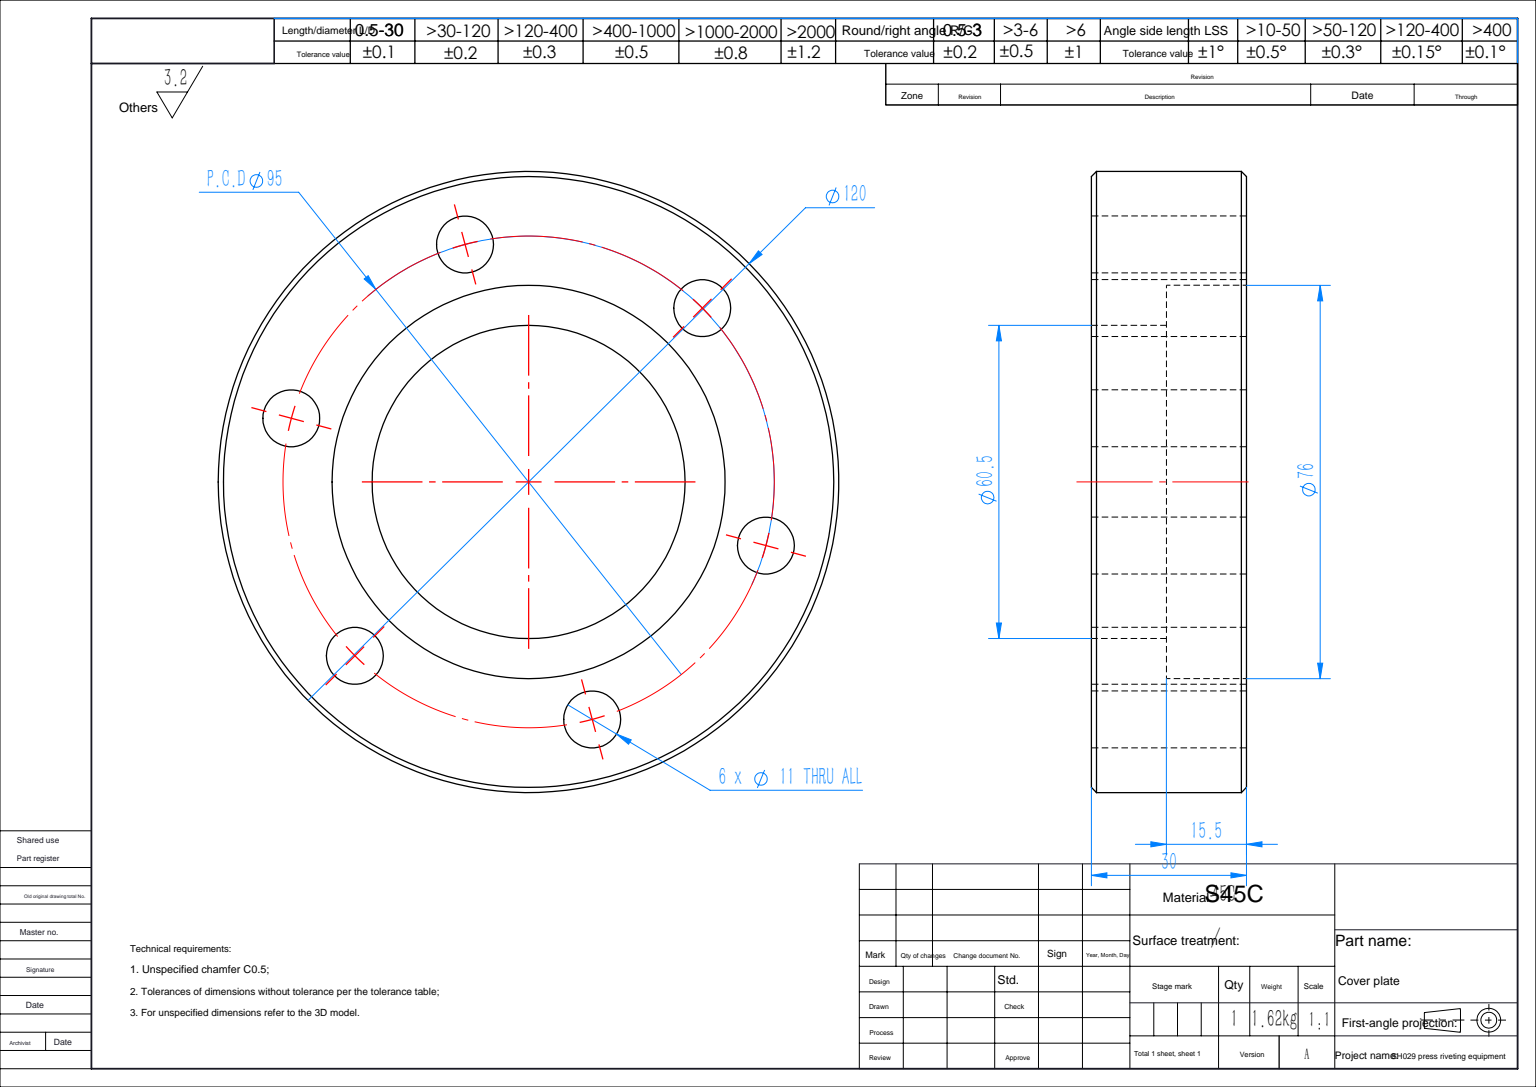
from build123d import *

# Parameters (mm, degrees)
CHAMFER_1_SIZE           = 1
HOLE_WIZARD_M10_1_D      = 11
PATTERN_CIRCULAR_1_COUNT = 6


with BuildPart() as part:
    # 草图1 → 旋转1 (revolve)
    with BuildSketch(Plane(origin=(0, 0, 0), x_dir=(1, 0, 0), z_dir=(0, 1, 0)), mode=Mode.PRIVATE) as revolve_1_sk:
        Polygon((-15, 60), (15, 60), (15, 38), (-0.5, 38), (-0.5, 30.25), (-15, 30.25), align=None)
    revolve(revolve_1_sk.sketch.rotate(Axis((-222.715084562, 0, 0), (1, 0, 0)), 180), axis=Axis((-222.715084562, 0, 0), (1, 0, 0)))

    # 倒角1
    chamfer_1_edges = [part.edges().sort_by_distance(p)[0] for p in [
        (15, 0, -60),
        (-15, 0, -60),
    ]]
    chamfer(chamfer_1_edges, length=CHAMFER_1_SIZE)

    # M10 间隙孔1 (through all)
    with Locations(Plane.ZY.offset(15)):
        with Locations((33.587572106, -33.587572106)):
            hole_wizard_m10_1 = Hole(HOLE_WIZARD_M10_1_D / 2)

    # 阵列(圆周)1: M10 间隙孔1 ×6 about axis
    pattern_circular_1_axis = Axis((0, 0, 0), (1, 0, 0))
    for i in range(1, PATTERN_CIRCULAR_1_COUNT):
        add(hole_wizard_m10_1.rotate(pattern_circular_1_axis, i * 360 / PATTERN_CIRCULAR_1_COUNT), mode=Mode.SUBTRACT)


solid = part.part
